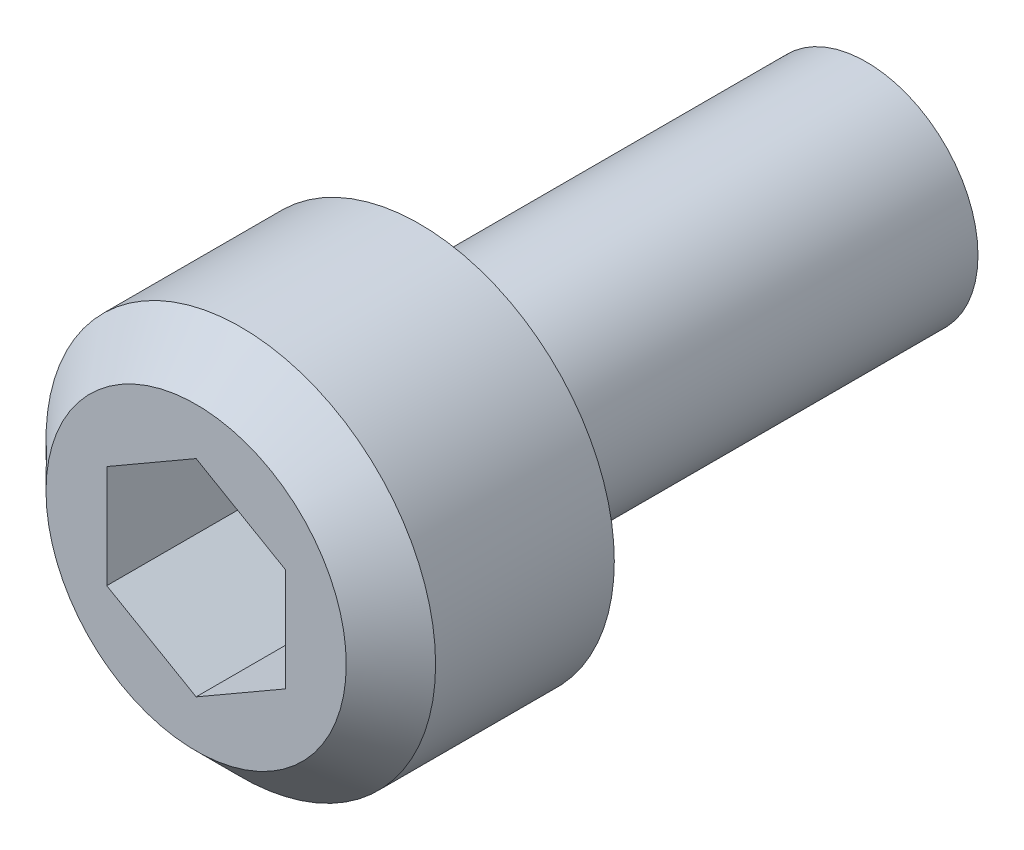
SolidWorks part; units mm, degrees
ref_plane "前视基准面" through (0, 0, 0) normal (0, 0, 1) x (1, 0, 0)
ref_plane "上视基准面" through (0, 0, 0) normal (0, 1, 0) x (1, 0, 0)
ref_plane "右视基准面" through (0, 0, 0) normal (1, 0, 0) x (0, 0, -1)
sketch "草图1" plane through (0, 0, 0) normal (0, 0, 1) x (1, 0, 0)
  circle A0 centre (0, 0) radius 4.36
  dimension "D1" = 8.72
extrude "凸台-拉伸1" add sketch "草图1" along normal blind 5
sketch "草图2" plane through (0, 0, 5) normal (0, 0, 1) x (1, 0, 0)
  line L1 (0, 2.3094) -> (-2, 1.1547)
  line L2 (-2, 1.1547) -> (-2, -1.1547)
  line L3 (-2, -1.1547) -> (0, -2.3094)
  line L4 (0, -2.3094) -> (2, -1.1547)
  line L5 (2, -1.1547) -> (2, 1.1547)
  line L6 (2, 1.1547) -> (0, 2.3094)
  circle A0 centre (0, 0) radius 2 construction
  dimension "D1" = 4
extrude "切除-拉伸1" cut sketch "草图2" against normal blind 4
chamfer "倒角1" distance 1 angle 45 1 edges at (4.36, 0, 5)
sketch "草图3" plane through (0, 0, 0) normal (0, 0, -1) x (-1, 0, 0)
  circle A0 centre (0, 0) radius 2.5
  dimension "D1" = 5
extrude "凸台-拉伸2" add sketch "草图3" along normal blind 10
cosmetic thread "装饰螺纹线1" parameters "D2"=4.917
